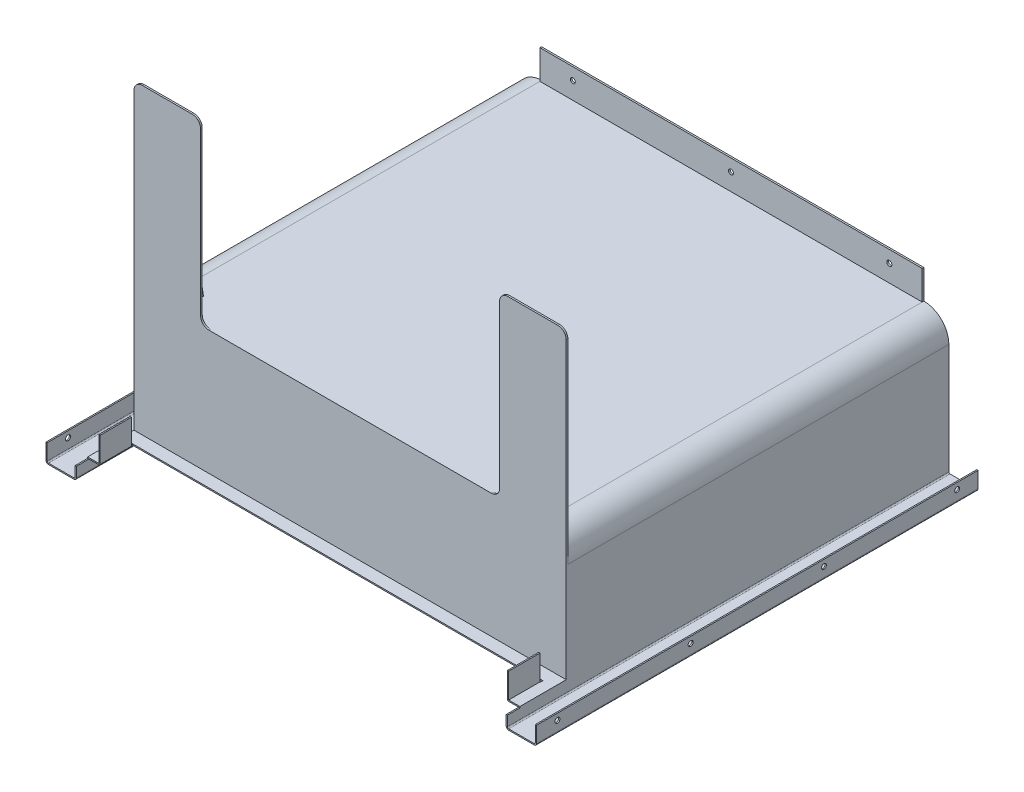
SolidWorks part; units mm, degrees
ref_plane "前视" through (0, 0, 0) normal (0, 0, 1) x (1, 0, 0)
ref_plane "上视" through (0, 0, 0) normal (0, 1, 0) x (1, 0, 0)
ref_plane "右视" through (0, 0, 0) normal (1, 0, 0) x (0, 0, -1)
sketch "草图1" plane through (0, 0, 0) normal (0, 0, 1) x (1, 0, 0)
  line L0 (-261, -82) -> (-293, -82)
  line L1 (-293, -82) -> (-293, -61.5)
  line L2 (259.5, -80.5) -> (259.5, 52)
  line L3 (229.5, 82) -> (-229.5, 82)
  line L4 (-259.5, -80.5) -> (-259.5, 52)
  line L5 (259.5, -82) -> (-259.5, 82) construction
  line L6 (259.5, 82) -> (-259.5, -82) construction
  line L7 (261, -82) -> (293, -82)
  line L8 (293, -82) -> (293, -61.5)
  arc A0 (261, -82) -> (259.5, -80.5) centre (261, -80.5) cw
  arc A1 (-261, -82) -> (-259.5, -80.5) centre (-261, -80.5) ccw
  arc A2 (259.5, 52) -> (229.5, 82) centre (229.5, 52) ccw
  arc A3 (-229.5, 82) -> (-259.5, 52) centre (-229.5, 52) ccw
  point P0 (0, 0)
  dimension "D4" = 1.5
  dimension "D5" = 30
  dimension "D1" = 586
  dimension "D2" = 519
  dimension "D3" = 164
  dimension "D6" = 20.5
  dimension "D7" = 20.5
extrude "拉伸-薄壁1" add sketch "草图1" along normal blind 530 thin thin type one direction wall 1.5
fillet "圆角1" radius 3 2 edges at (294.5, -83.5, 265) (-294.5, -83.5, 265)
fillet "圆角6" radius 1.5 2 edges at (-293, -82, 265) (293, -82, 265)
sketch "草图2" plane through (0, 0, 530) normal (0, 0, 1) x (1, 0, 0)
  line L0 (261, -83.5) -> (291.5, -83.5) construction
  line L1 (-330.6279, 139.2518) -> (320.671, 139.2518)
  line L2 (-330.6279, 139.2518) -> (-330.6279, -68.5)
  line L3 (-330.6279, -68.5) -> (320.671, -68.5)
  line L4 (320.671, 139.2518) -> (320.671, -68.5)
  dimension "D1" = 15
extrude "切除-拉伸1" cut sketch "草图2" against normal blind 72.6
sketch "草图3" plane through (0, 0, 457.4) normal (0, 0, 1) x (1, 0, 0)
  line L0 (259.5, 52) -> (259.5, -68.5) construction
  line L1 (-259.5, 287.1) -> (259.5, 287.1) construction
  line L2 (-259.5, 287.1) -> (-259.5, -68.5) construction
  line L3 (-259.5, -68.5) -> (259.5, -68.5) construction
  line L4 (259.5, 287.1) -> (259.5, -68.5) construction
  line L7 (-259.5, -68.5) -> (-259.5, 52) construction
  dimension "D2" = 355.6
sketch "草图4" plane through (0, 0, 457.4) normal (0, 0, 1) x (1, 0, 0)
  line L1 (-259.5, 296.5) -> (259.5, 296.5)
  line L2 (-259.5, 296.5) -> (-259.5, -68.5)
  line L3 (-259.5, -68.5) -> (259.5, -68.5)
  line L4 (259.5, 296.5) -> (259.5, -68.5)
  dimension "D1" = 365
extrude "凸台-拉伸10" add sketch "草图4" along normal blind 2 separate body
sketch "草图5" plane through (0, 0, 459.4) normal (0, 0, 1) x (1, 0, 0)
  line L0 (0, 295.6694) -> (0, -122.0684) construction
  line L1 (259.5, 296.5) -> (-259.5, 296.5) construction
  line L2 (-179.5, 296.5) -> (179.5, 296.5)
  line L3 (-179.5, 296.5) -> (-179.5, 82)
  line L4 (-179.5, 82) -> (179.5, 82)
  line L5 (179.5, 296.5) -> (179.5, 82)
  line L6 (-259.5, 296.5) -> (-259.5, -68.5) construction
  line L7 (-229.5, 82) -> (229.5, 82) construction
  point P9 (0, 82)
  dimension "D1" = 80
extrude "切除-拉伸2" cut sketch "草图5" against normal through all
fillet "圆角2" radius 10 1 edges at (179.5, 82, 458.4)
fillet "圆角3" radius 10 1 edges at (-179.5, 82, 458.4)
ref_plane "基准面1" through (-209.5, 0, 0) normal (1, 0, 0) x (0, 0, -1)
sketch "草图6" plane through (-209.5, 0, 0) normal (1, 0, 0) x (0, 0, -1)
  line L0 (-457.4, 276.5) -> (-427.4, 82)
  line L1 (-457.4, 287.1) -> (-457.4, -68.5) construction
  line L3 (-427.4, 82) -> (-457.4, 82)
  line L4 (-457.4, 82) -> (-457.4, 276.5)
  line L5 (-459.4, 296.5) -> (-457.4, 296.5) construction
  line L6 (-457.4, 82) -> (0, 82) construction
  dimension "D1" = 20
  dimension "D2" = 30
extrude "凸台-拉伸13" add sketch "草图6" along normal mid plane 3 separate body
ref_plane "基准面2" through (209.5, 0, 0) normal (-1, 0, 0) x (0, 0, 1)
sketch "草图8" plane through (209.5, 0, 0) normal (-1, 0, 0) x (0, 0, 1)
  line L0 (457.4, 276.5) -> (427.4, 82)
  line L1 (457.4, 287.1) -> (457.4, -68.5) construction
  line L2 (457.4, 82) -> (0, 82) construction
  line L3 (427.4, 82) -> (457.4, 82)
  line L4 (457.4, 82) -> (457.4, 276.5)
  line L5 (459.4, 296.5) -> (457.4, 296.5) construction
  dimension "D1" = 20
  dimension "D2" = 30
extrude "凸台-拉伸14" add sketch "草图8" along normal blind 3 separate body
fillet "圆角4" radius 10 4 edges at (-179.5, 296.5, 458.4) (-259.5, 296.5, 458.4) (179.5, 296.5, 458.4) (259.5, 296.5, 458.4)
sketch "草图9" plane through (0, -68.5, 0) normal (0, -1, 0) x (1, 0, 0)
  line L4 (-259.5, 457.4) -> (259.5, 457.4)
  line L5 (259.5, 457.4) -> (259.5, 459.4)
  line L6 (259.5, 459.4) -> (-259.5, 459.4)
  line L7 (259.5, 457.4) -> (259.5, 459.4)
  line L8 (-259.5, 457.4) -> (259.5, 457.4)
  line L9 (-259.5, 459.4) -> (-259.5, 457.4)
  line L10 (259.5, 459.4) -> (-259.5, 459.4)
  line L11 (-259.5, 459.4) -> (-259.5, 457.4)
  dimension "D1" = 0
sketch "草图10" plane through (0, 0, 0) normal (0, 0, -1) x (-1, 0, 0)
  line L0 (-294.5, -61.5) -> (-294.5, 82)
  line L1 (294.5, -61.5) -> (294.5, 81.671)
  line L2 (229.5, 82) -> (294.5, 81.671)
  line L3 (-229.5, 82) -> (-294.5, 82)
  line L16 (-294.5, -61.5) -> (-294.5, -80.5)
  line L17 (-291.5, -83.5) -> (-261, -83.5)
  line L18 (-258, -80.5) -> (-258, 52)
  line L19 (-229.5, 80.5) -> (229.5, 80.5)
  line L20 (258, 52) -> (258, -80.5)
  line L21 (261, -83.5) -> (291.5, -83.5)
  line L22 (294.5, -80.5) -> (294.5, -61.5)
  line L23 (294.5, -61.5) -> (293, -61.5)
  line L24 (293, -61.5) -> (293, -80.5)
  line L25 (291.5, -82) -> (261, -82)
  line L26 (259.5, -80.5) -> (259.5, 52)
  line L27 (229.5, 82) -> (-229.5, 82)
  line L28 (-259.5, 52) -> (-259.5, -80.5)
  line L29 (-261, -82) -> (-291.5, -82)
  line L30 (-293, -80.5) -> (-293, -61.5)
  line L31 (-293, -61.5) -> (-294.5, -61.5)
  line L32 (-294.5, -61.5) -> (-294.5, -80.5)
  line L33 (-291.5, -83.5) -> (-261, -83.5)
  line L34 (-258, -80.5) -> (-258, 52)
  line L35 (-229.5, 80.5) -> (229.5, 80.5)
  line L36 (258, 52) -> (258, -80.5)
  line L37 (261, -83.5) -> (291.5, -83.5)
  line L38 (294.5, -80.5) -> (294.5, -61.5)
  line L43 (229.5, 82) -> (-229.5, 82)
  arc A10 (-294.5, -80.5) -> (-291.5, -83.5) centre (-291.5, -80.5) ccw
  arc A11 (-261, -83.5) -> (-258, -80.5) centre (-261, -80.5) ccw
  arc A12 (-229.5, 80.5) -> (-258, 52) centre (-229.5, 52) ccw
  arc A13 (258, 52) -> (229.5, 80.5) centre (229.5, 52) ccw
  arc A14 (258, -80.5) -> (261, -83.5) centre (261, -80.5) ccw
  arc A15 (291.5, -83.5) -> (294.5, -80.5) centre (291.5, -80.5) ccw
  arc A16 (259.5, -80.5) -> (261, -82) centre (261, -80.5) ccw
  arc A17 (259.5, 52) -> (229.5, 82) centre (229.5, 52) ccw
  arc A18 (-229.5, 82) -> (-259.5, 52) centre (-229.5, 52) ccw
  arc A19 (-261, -82) -> (-259.5, -80.5) centre (-261, -80.5) ccw
  arc A20 (-294.5, -80.5) -> (-291.5, -83.5) centre (-291.5, -80.5) ccw
  arc A21 (-261, -83.5) -> (-258, -80.5) centre (-261, -80.5) ccw
  arc A22 (-229.5, 80.5) -> (-258, 52) centre (-229.5, 52) ccw
  arc A23 (258, 52) -> (229.5, 80.5) centre (229.5, 52) ccw
  arc A24 (258, -80.5) -> (261, -83.5) centre (261, -80.5) ccw
  arc A25 (291.5, -83.5) -> (294.5, -80.5) centre (291.5, -80.5) ccw
  arc A28 (291.5, -82) -> (293, -80.5) centre (291.5, -80.5) ccw
  arc A29 (291.5, -82) -> (293, -80.5) centre (291.5, -80.5) ccw
  arc A30 (-293, -80.5) -> (-291.5, -82) centre (-291.5, -80.5) ccw
  arc A31 (-293, -80.5) -> (-291.5, -82) centre (-291.5, -80.5) ccw
  dimension "D1" = 0
sketch "草图13" plane through (0, -68.5, 0) normal (0, 1, 0) x (1, 0, 0)
  line L0 (259.5, -530) -> (259.5, -457.4) construction
  line L1 (259.5, -515) -> (-259.5, -515)
  line L2 (259.5, -515) -> (259.5, -459.4)
  line L3 (259.5, -459.4) -> (-259.5, -459.4)
  line L4 (-259.5, -515) -> (-259.5, -459.4)
  line L5 (258, -530) -> (259.5, -530) construction
  point P8 (258.75, -530)
  dimension "D1" = 15
extrude "凸台-拉伸15" add sketch "草图13" along normal blind 1.5
sketch "草图14" plane through (0, -67, 0) normal (0, 1, 0) x (1, 0, 0)
  line L0 (-259.5, -515) -> (259.5, -515) construction
  line L1 (244.5, -515) -> (-244.5, -515)
  line L2 (244.5, -515) -> (244.5, -474.4)
  line L3 (244.5, -474.4) -> (-244.5, -474.4)
  line L4 (-244.5, -515) -> (-244.5, -474.4)
  line L5 (259.5, -515) -> (259.5, -459.4) construction
  line L6 (259.5, -459.4) -> (-259.5, -459.4) construction
  line L7 (-259.5, -530) -> (-259.5, 0) construction
  dimension "D1" = 15
  dimension "D2" = 15
  dimension "D3" = 15
extrude "切除-拉伸5" cut sketch "草图14" against normal blind 1.5
sketch "草图15" plane through (0, -67, 0) normal (0, 1, 0) x (1, 0, 0)
  line L0 (244.5, -474.4) -> (-244.5, -474.4) construction
  line L1 (244.5, -515) -> (246, -515)
  line L2 (244.5, -515) -> (244.5, -477.4)
  line L3 (244.5, -477.4) -> (246, -477.4)
  line L4 (246, -515) -> (246, -477.4)
  line L5 (-244.5, -515) -> (-246, -515)
  line L6 (-244.5, -515) -> (-244.5, -477.4)
  line L7 (-244.5, -477.4) -> (-246, -477.4)
  line L8 (-246, -515) -> (-246, -477.4)
  dimension "D1" = 1.5
  dimension "D2" = 3
extrude "凸台-拉伸16" add sketch "草图15" along normal blind 30
sketch "草图16" plane through (0, -67, 0) normal (0, 1, 0) x (1, 0, 0)
  line L0 (244.5, -474.4) -> (-244.5, -474.4) construction
  line L1 (244.5, -477.4) -> (246.5, -477.4)
  line L2 (244.5, -477.4) -> (244.5, -474.4)
  line L3 (244.5, -474.4) -> (246.5, -474.4)
  line L4 (246.5, -477.4) -> (246.5, -474.4)
  line L6 (-244.5, -477.4) -> (-246.5, -477.4)
  line L7 (-244.5, -477.4) -> (-244.5, -474.4)
  line L8 (-244.5, -474.4) -> (-246.5, -474.4)
  line L9 (-246.5, -477.4) -> (-246.5, -474.4)
  dimension "D1" = 2
extrude "切除-拉伸6" cut sketch "草图16" against normal blind 2
fillet "圆角5" radius 1.5 2 edges at (-244.5, -68.5, 496.2) (244.5, -68.5, 496.2)
sketch "草图17" plane through (0, 0, 0) normal (0, 0, -1) x (-1, 0, 0)
  line L1 (-229.5, 82) -> (229.5, 82)
  line L2 (-229.5, 82) -> (-229.5, 117)
  line L3 (-229.5, 117) -> (229.5, 117)
  line L4 (229.5, 82) -> (229.5, 117)
  dimension "D1" = 35
extrude "凸台-拉伸17" add sketch "草图17" against normal blind 2
hole_wizard "Ø6.0 (6) 直径孔1" positions "草图19" profile "草图18" hole size "Ø6.0" standard "Ansi Metric" end condition through all
sketch "草图19" plane through (0, 0, 2) normal (0, 0, 1) x (1, 0, 0)
  line L0 (0, 117) -> (0, 88) construction
  line L1 (-229.5, 117) -> (229.5, 117) construction
  point P0 (-190, 102.5)
  point P2 (0, 102.5)
  point P4 (190, 102.5)
  dimension "D1" = 380
  dimension "D2" = 14.5
sketch "草图18" plane through (-190, 102.5, 2) normal (1, 0, 0) x (0, -1, 0)
  line L0 (0, 0) -> (0, 2)
  line L1 (0, 2) -> (3, 2)
  line L2 (3, 2) -> (3, 0)
  line L5 (3, 0) -> (0, 0)
  line L11 (0, -6.35) -> (0, 107.95) construction
  dimension "通孔孔直径" = 6
  dimension "通孔孔深度" = 2
sketch "草图20" plane through (0, 0, 457.4) normal (0, 0, 1) x (1, 0, 0)
  line L1 (293, -68.5) -> (294.5, -68.5)
  line L2 (293, -68.5) -> (293, -61.5)
  line L3 (293, -61.5) -> (294.5, -61.5)
  line L4 (294.5, -68.5) -> (294.5, -61.5)
  line L5 (-293, -68.5) -> (-294.5, -68.5)
  line L6 (-293, -68.5) -> (-293, -61.5)
  line L7 (-293, -61.5) -> (-294.5, -61.5)
  line L8 (-294.5, -68.5) -> (-294.5, -61.5)
extrude "凸台-拉伸18" add sketch "草图20" along normal up to surface (72.6 mm away) up to face at (-276.25, -77.4053, 530)
hole_wizard "Ø6.0 (6) 直径孔2" positions "草图22" profile "草图21" hole size "Ø6.0" standard "Gb"
sketch "草图22" plane through (294.5, 0, 0) normal (1, 0, 0) x (0, 0, -1)
  line L0 (-265, -61.5) -> (-265, -97.6184) construction
  line L1 (-530, -61.5) -> (0, -61.5) construction
  point P0 (-505, -69)
  point P2 (-345, -69)
  point P4 (-185, -69)
  point P6 (-25, -69)
  dimension "D1" = 160
  dimension "D2" = 160
  dimension "D3" = 7.5
sketch "草图21" plane through (294.5, -69, 505) normal (0, 1, 0) x (0, 0, -1)
  line L0 (0, 0) -> (0, 3.8026)
  line L1 (0, 3.8026) -> (3, 2)
  line L2 (3, 2) -> (3, 0)
  line L5 (3, 0) -> (0, 0)
  line L10 (0, 3.8026) -> (-3, 2) construction
  line L11 (0, -6.35) -> (0, 107.95) construction
  dimension "孔直径" = 6
  dimension "孔深度" = 2
  dimension "导头角度" = 118
hole_wizard "Ø6.0 (6) 直径孔3" positions "草图24" profile "草图23" hole size "Ø6.0" standard "Gb"
sketch "草图24" plane through (-294.5, 0, 0) normal (-1, 0, 0) x (0, 0, 1)
  point P0 (25, -69)
  point P2 (185, -69)
  point P4 (345, -69)
  point P6 (505, -69)
sketch "草图23" plane through (-294.5, -69, 25) normal (0, 1, 0) x (0, 0, 1)
  line L0 (0, 0) -> (0, 3.8026)
  line L1 (0, 3.8026) -> (3, 2)
  line L2 (3, 2) -> (3, 0)
  line L5 (3, 0) -> (0, 0)
  line L10 (0, 3.8026) -> (-3, 2) construction
  line L11 (0, -6.35) -> (0, 107.95) construction
  dimension "孔直径" = 6
  dimension "孔深度" = 2
  dimension "导头角度" = 118
